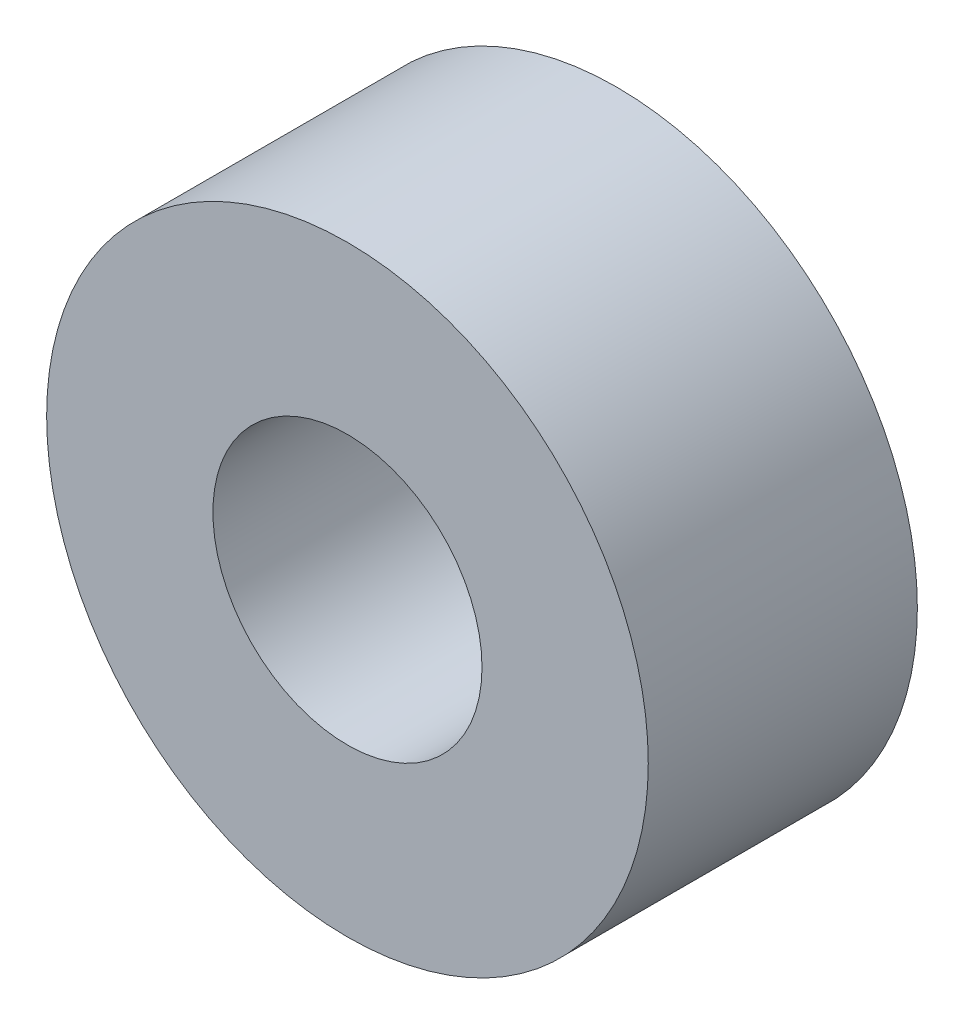
from build123d import *

# Parameters (mm, degrees)
SKETCH1_R           = 5.589643184
SKETCH1_R_2         = 2.5
BOSS_EXTRUDE1_DEPTH = 5


with BuildPart() as part:
    # Sketch1 → Boss-Extrude1 (new body)
    with BuildSketch(Plane.XY):
        Circle(SKETCH1_R)
        Circle(SKETCH1_R_2, mode=Mode.SUBTRACT)
    extrude(amount=BOSS_EXTRUDE1_DEPTH)


solid = part.part
